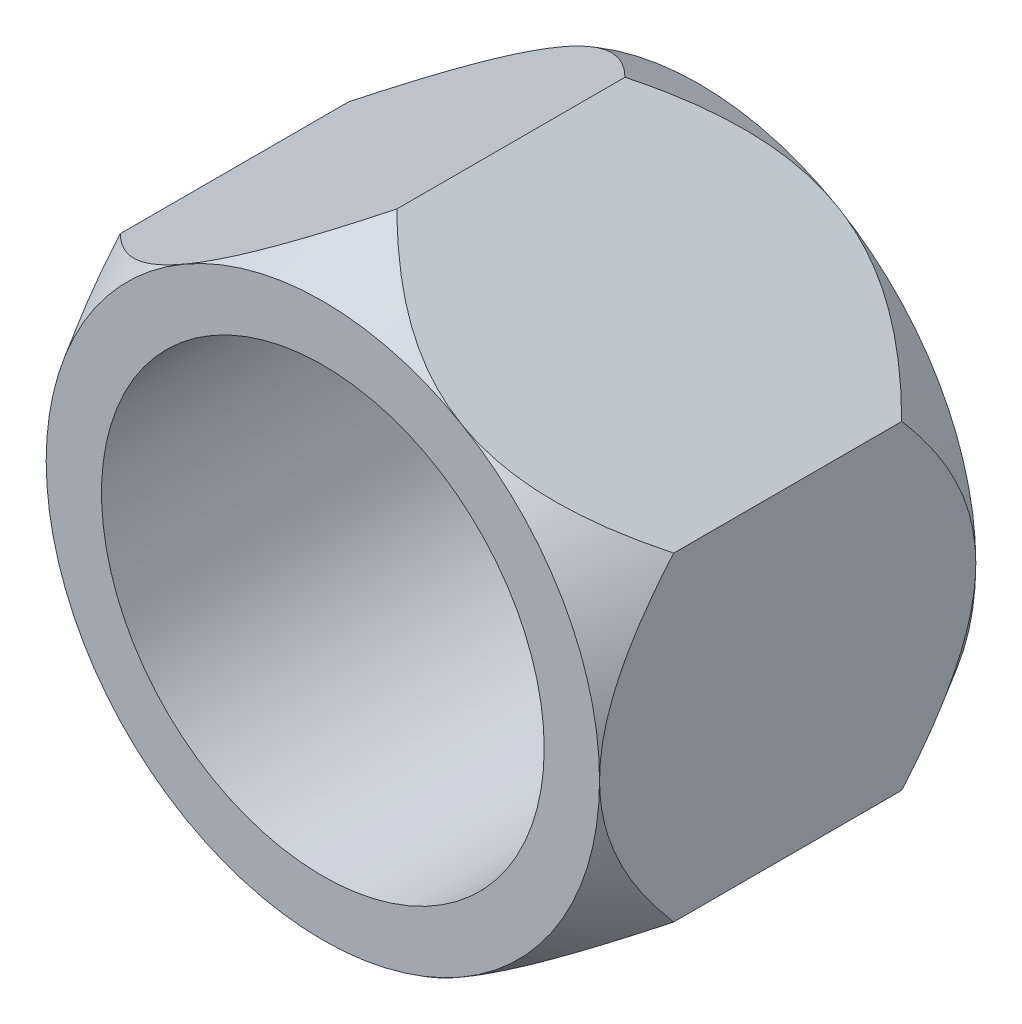
from build123d import *

# Parameters (mm, degrees)
BOSS_EXTRUDE1_DEPTH     = 3.4
SKETCH2_OUTSIDE_W       = 23.196
SKETCH2_OUTSIDE_H       = 24.744
SKETCH2_OUTSIDE_R       = 5
CUT_EXTRUDE1_DEPTH      = 6.8
CUT_EXTRUDE1_DRAFT      = -30
MIRROR1_COPY_1_SKETCH_W = 23.196
MIRROR1_COPY_1_SKETCH_H = 24.744
MIRROR1_COPY_1_SKETCH_R = 5
MIRROR1_COPY_1_DEPTH    = 6.8
MIRROR1_COPY_1_DRAFT    = -30
SKETCH3_R               = 4
CUT_EXTRUDE3_DEPTH      = 6.8


with BuildPart() as part:
    # Sketch1 → Boss-Extrude1 (new, symmetric)
    with BuildSketch(Plane.XY):
        Polygon((0, 5.773502692), (-5, 2.886751346), (-5, -2.886751346), (0, -5.773502692), (5, -2.886751346), (5, 2.886751346), align=None)
    extrude(amount=BOSS_EXTRUDE1_DEPTH, both=True)


with BuildPart() as cut_extrude1_tool:
    # Sketch2 outside → Cut-Extrude1 (with draft: the straight prism first)
    with BuildSketch(Plane.XY.offset(3.4)):
        Rectangle(SKETCH2_OUTSIDE_W, SKETCH2_OUTSIDE_H)
        Circle(SKETCH2_OUTSIDE_R, mode=Mode.SUBTRACT)
    extrude(amount=-CUT_EXTRUDE1_DEPTH)
    # Cut-Extrude1: the draft: its side faces are tilted about the plane it starts from
    cut_extrude1_sides = [cut_extrude1_tool.faces().sort_by_distance(p)[0] for p in [
        (0, -12.372, 0),
        (11.598, 0, 0),
        (0, 12.372, 0),
        (-11.598, 0, 0),
        (-5, 0, 0),
    ]]
    draft(cut_extrude1_sides, Plane.XY.offset(3.4), CUT_EXTRUDE1_DRAFT)


with BuildPart() as part_1:
    add(part.part)

    # Cut-Extrude1: cut by cut_extrude1_tool
    add(cut_extrude1_tool.part, mode=Mode.SUBTRACT)


with BuildPart() as mirror1_copy_1_tool:
    # Mirror1 copy 1 sketch → Mirror1 copy 1 (with draft: the straight prism first)
    with BuildSketch(Plane(origin=(0, 0, -3.4), x_dir=(1, 0, 0), z_dir=(0, 0, -1))):
        Rectangle(MIRROR1_COPY_1_SKETCH_W, MIRROR1_COPY_1_SKETCH_H)
        Circle(MIRROR1_COPY_1_SKETCH_R, mode=Mode.SUBTRACT)
    extrude(amount=-MIRROR1_COPY_1_DEPTH)
    # Mirror1 copy 1: the draft: its side faces are tilted about the plane it starts from
    mirror1_copy_1_sides = [mirror1_copy_1_tool.faces().sort_by_distance(p)[0] for p in [
        (0, -12.372, 0),
        (11.598, 0, 0),
        (0, 12.372, 0),
        (-11.598, 0, 0),
        (-5, 0, 0),
    ]]
    draft(mirror1_copy_1_sides, Plane(origin=(0, 0, -3.4), x_dir=(1, 0, 0), z_dir=(0, 0, -1)), MIRROR1_COPY_1_DRAFT)


with BuildPart() as part_2:
    add(part_1.part)

    # Mirror1 copy 1: cut by mirror1_copy_1_tool
    add(mirror1_copy_1_tool.part, mode=Mode.SUBTRACT)

    # Sketch3 → Cut-Extrude3 (cut)
    with BuildSketch(Plane.XY.offset(3.4)):
        Circle(SKETCH3_R)
    extrude(amount=-CUT_EXTRUDE3_DEPTH, mode=Mode.SUBTRACT)


solid = part_2.part
